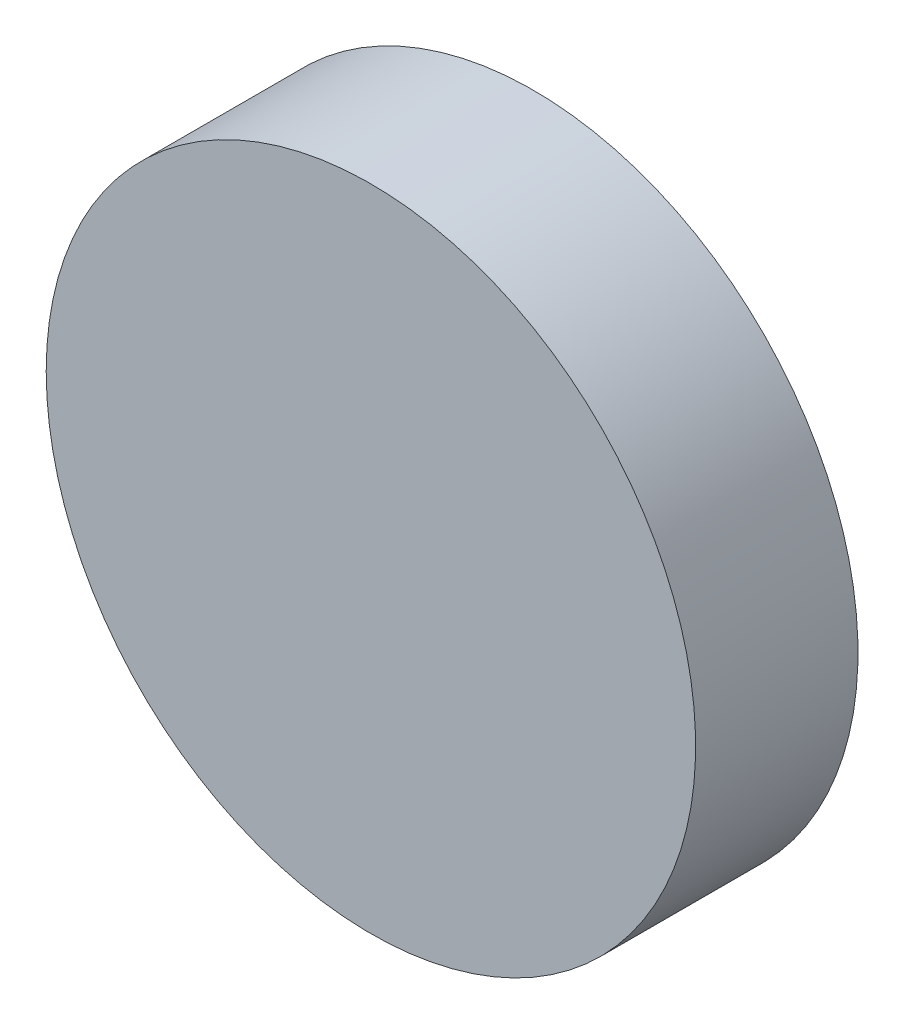
from build123d import *

# Parameters (mm, degrees)
SKETCH1_R           = 19.05
BOSS_EXTRUDE1_DEPTH = 9.525


with BuildPart() as part:
    # Sketch1 → Boss-Extrude1 (new body)
    with BuildSketch(Plane.XY):
        with Locations(Location((0, 0, 0), (0, 0, 180))):
            Circle(SKETCH1_R)
    extrude(amount=BOSS_EXTRUDE1_DEPTH)


solid = part.part
